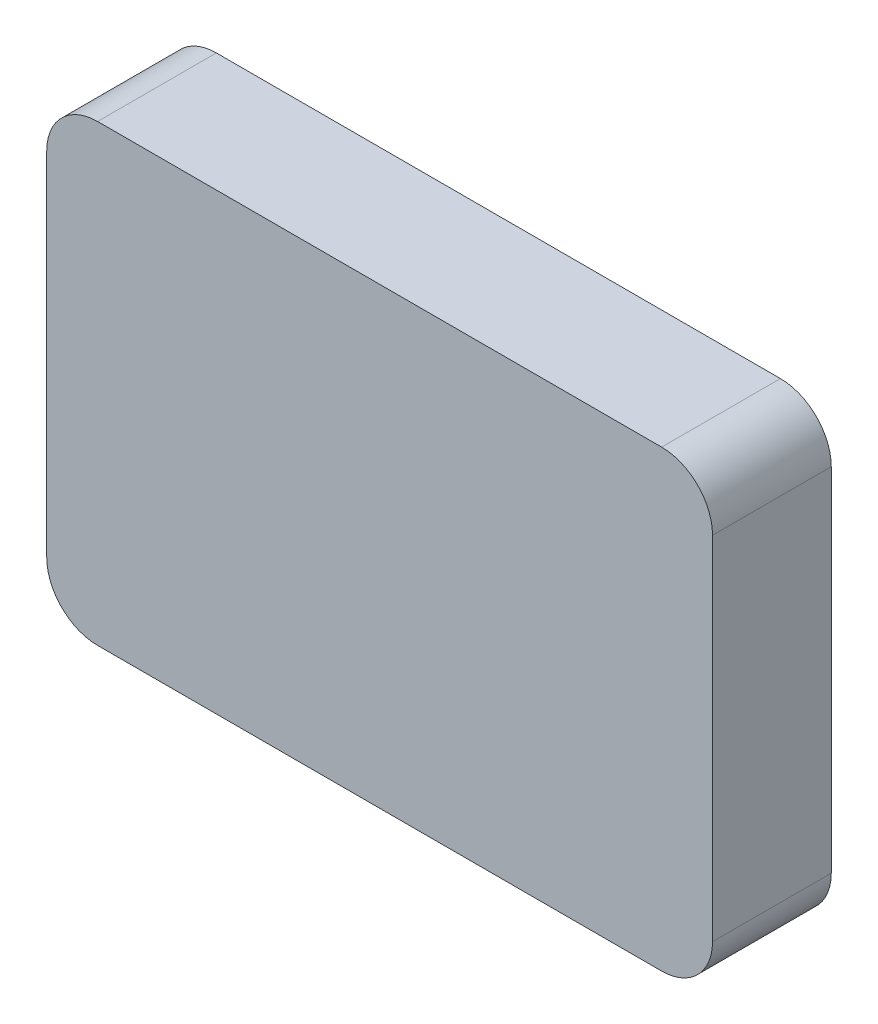
from build123d import *

# Parameters (mm, degrees)
SKETCH_1_W      = 78.5
SKETCH_1_H      = 53.5
EXTRUDE_1_DEPTH = 14
FILLET_1_R      = 6


with BuildPart() as part:
    # 草图1 → 凸台-拉伸1 (new body)
    with BuildSketch(Plane.XY):
        with Locations((39.25, 26.75)):
            Rectangle(SKETCH_1_W, SKETCH_1_H)
    extrude(amount=EXTRUDE_1_DEPTH)

    # 圆角1
    fillet_1_edges = [part.edges().sort_by_distance(p)[0] for p in [
        (0, 53.5, 7),
        (78.5, 53.5, 7),
        (78.5, 0, 7),
        (0, 0, 7),
    ]]
    fillet(fillet_1_edges, radius=FILLET_1_R)


solid = part.part
